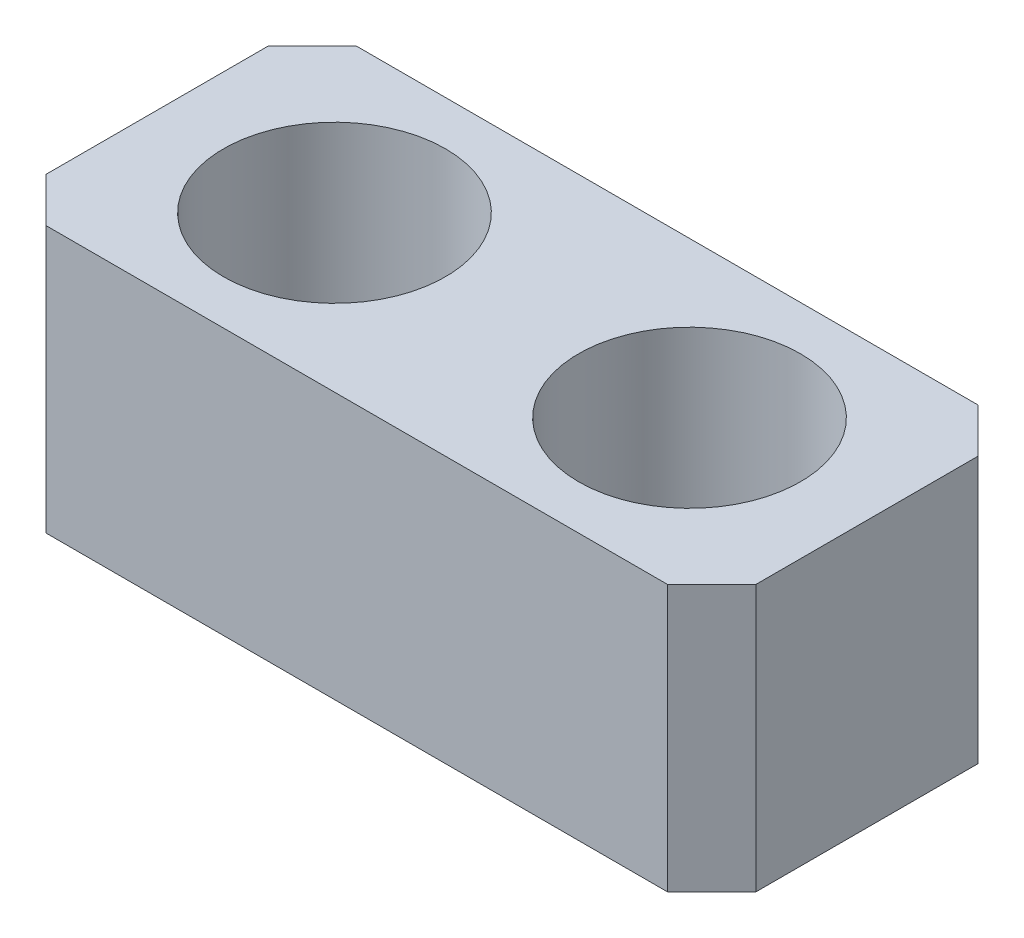
from build123d import *

# Parameters (mm, degrees)
SKETCH1_W                  = 8
SKETCH1_H                  = 3.5
BOSS_EXTRUDE1_DEPTH        = 1.5
SKETCH2_R                  = 1.25
CUT_EXTRUDE1_DEPTH         = 2
CHAMFER1_SIZE              = 0.5
F_1_0_1_DIAMETER_HOLE1_D   = 1
F_2_5_2_5_DIAMETER_HOLE1_D = 2.5


with BuildPart() as part:
    # Sketch1 → Boss-Extrude1 (new, symmetric)
    with BuildSketch(Plane(origin=(0, 0, 0), x_dir=(1, 0, 0), z_dir=(0, 1, 0))):
        Rectangle(SKETCH1_W, SKETCH1_H)
    extrude(amount=BOSS_EXTRUDE1_DEPTH, both=True)

    # Sketch2 → Cut-Extrude1 (cut)
    with BuildSketch(Plane(origin=(0, 1.5, 0), x_dir=(1, 0, 0), z_dir=(0, 1, 0))):
        with Locations(Location((-2, 0, 0), (0, 0, 270))):
            Circle(SKETCH2_R)
    extrude(amount=-CUT_EXTRUDE1_DEPTH, mode=Mode.SUBTRACT)

    # Chamfer1
    chamfer1_edges = [part.edges().sort_by_distance(p)[0] for p in [
        (4, 0, 1.75),
        (-4, 0, 1.75),
        (-4, 0, -1.75),
        (4, 0, -1.75),
    ]]
    chamfer(chamfer1_edges, length=CHAMFER1_SIZE)

    # Ø1.0 (1) Diameter Hole1 (through all)
    with Locations(Plane(origin=(0, -1.5, 0), x_dir=(-1, 0, 0), z_dir=(0, -1, 0))):
        with Locations((2, 0)):
            Hole(F_1_0_1_DIAMETER_HOLE1_D / 2)

    # Ø2.5 (2.5) Diameter Hole1 (through all)
    with Locations(Plane(origin=(0, -1.5, 0), x_dir=(-1, 0, 0), z_dir=(0, -1, 0))):
        with Locations((-2, 0)):
            Hole(F_2_5_2_5_DIAMETER_HOLE1_D / 2)


solid = part.part
